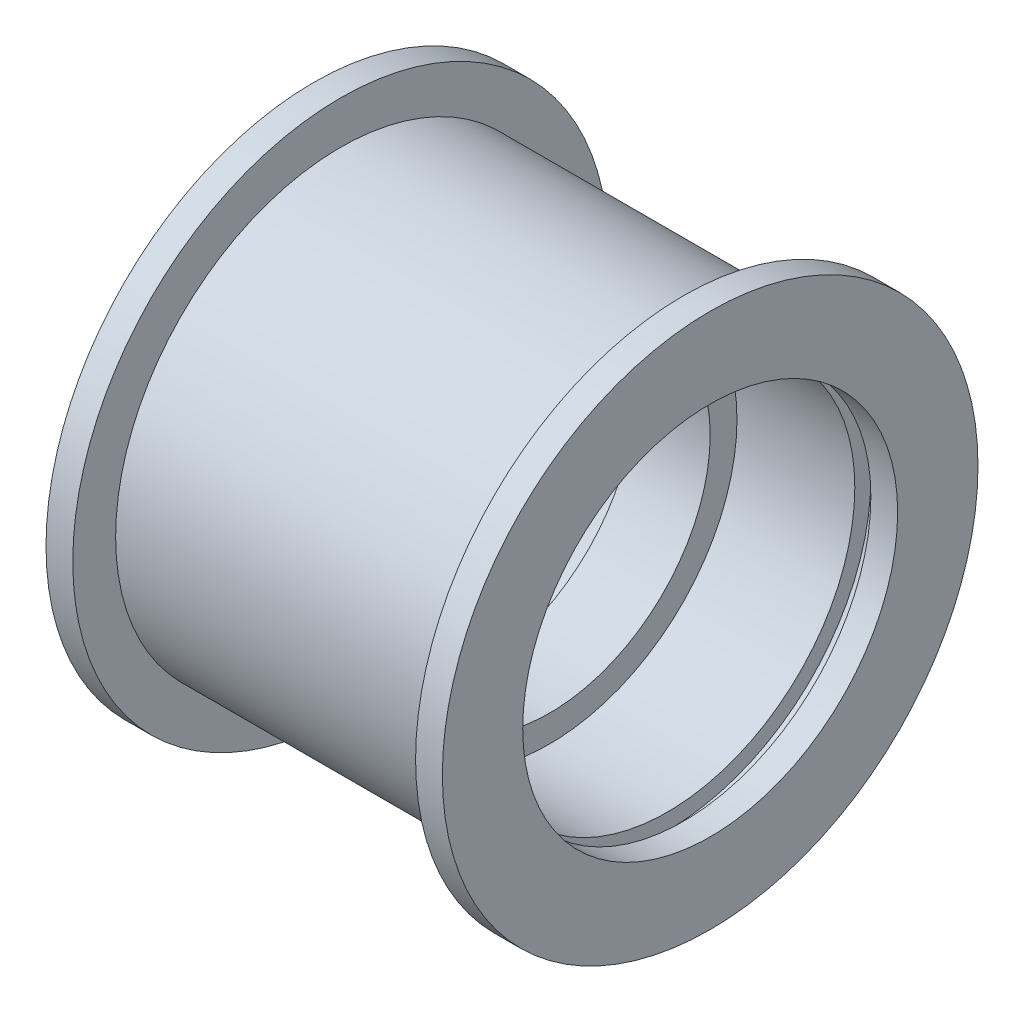
from build123d import *

# Parameters (mm, degrees)
SKETCH_1_R          = 21
EXTRUDE_1_DEPTH     = 16
SKETCH_6_R          = 25
EXTRUDE_2_DEPTH     = 1.5
SKETCH_7_R          = 25
EXTRUDE_3_DEPTH     = 1
SKETCH_8_R          = 15
CUT_EXTRUDE_1_DEPTH = 52.176166328
SKETCH_9_R          = 17.5
CUT_EXTRUDE_2_DEPTH = 15
SKETCH_10_W         = 1.5
SKETCH_10_H         = 1.5


with BuildPart() as part:
    # 草图1 → 拉伸1 (new, symmetric)
    with BuildSketch(Plane(origin=(0, 0, 0), x_dir=(0, 0, -1), z_dir=(1, 0, 0))):
        Circle(SKETCH_1_R)
    extrude(amount=EXTRUDE_1_DEPTH, both=True)

    # 草图6 → 凸台-拉伸2 (add)
    with BuildSketch(Plane(origin=(16, 0, 0), x_dir=(0, 0, -1), z_dir=(1, 0, 0))):
        Circle(SKETCH_6_R)
    extrude_2 = extrude(amount=EXTRUDE_2_DEPTH)

    # 草图7 → 凸台-拉伸3 (add)
    with BuildSketch(Plane(origin=(17.5, 0, 0), x_dir=(0, 0, -1), z_dir=(1, 0, 0))):
        Circle(SKETCH_7_R)
    extrude_3 = extrude(amount=EXTRUDE_3_DEPTH)

    # 镜向2: 凸台-拉伸2, 凸台-拉伸3 across plane
    add(extrude_2.mirror(Plane(origin=(0, 0, 0), x_dir=(0, 0, 1), z_dir=(1, 0, 0))))
    add(extrude_3.mirror(Plane(origin=(0, 0, 0), x_dir=(0, 0, 1), z_dir=(1, 0, 0))))

    # 草图8 → 切除-拉伸1 (cut, through all)
    with BuildSketch(Plane.ZY.offset(18.5)):
        Circle(SKETCH_8_R)
    extrude(amount=-CUT_EXTRUDE_1_DEPTH, mode=Mode.SUBTRACT)

    # 草图9 → Cut-Extrude 2 (cut)
    with BuildSketch(Plane.ZY.offset(18.5)):
        Circle(SKETCH_9_R)
    cut_extrude_2 = extrude(amount=-CUT_EXTRUDE_2_DEPTH, mode=Mode.SUBTRACT)

    # 草图10 → 切除-旋转1 (revolve, cut)
    with BuildSketch(Plane(origin=(0, 0, 0), x_dir=(1, 0, 0), z_dir=(0, 1, 0)), mode=Mode.PRIVATE) as cut_revolve_1_sk:
        with Locations((-15.25, 18.25)):
            Rectangle(SKETCH_10_W, SKETCH_10_H)
    cut_revolve_1 = revolve(cut_revolve_1_sk.sketch.rotate(Axis((0, 0, 0), (-1, 0, 0)), 180), axis=Axis((0, 0, 0), (-1, 0, 0)), mode=Mode.SUBTRACT)

    # 镜向3: Cut-Extrude 2, 切除-旋转1 across plane
    add(cut_extrude_2.mirror(Plane(origin=(0, 0, 0), x_dir=(0, 0, 1), z_dir=(1, 0, 0))), mode=Mode.SUBTRACT)
    add(cut_revolve_1.mirror(Plane(origin=(0, 0, 0), x_dir=(0, 0, 1), z_dir=(1, 0, 0))), mode=Mode.SUBTRACT)


solid = part.part
